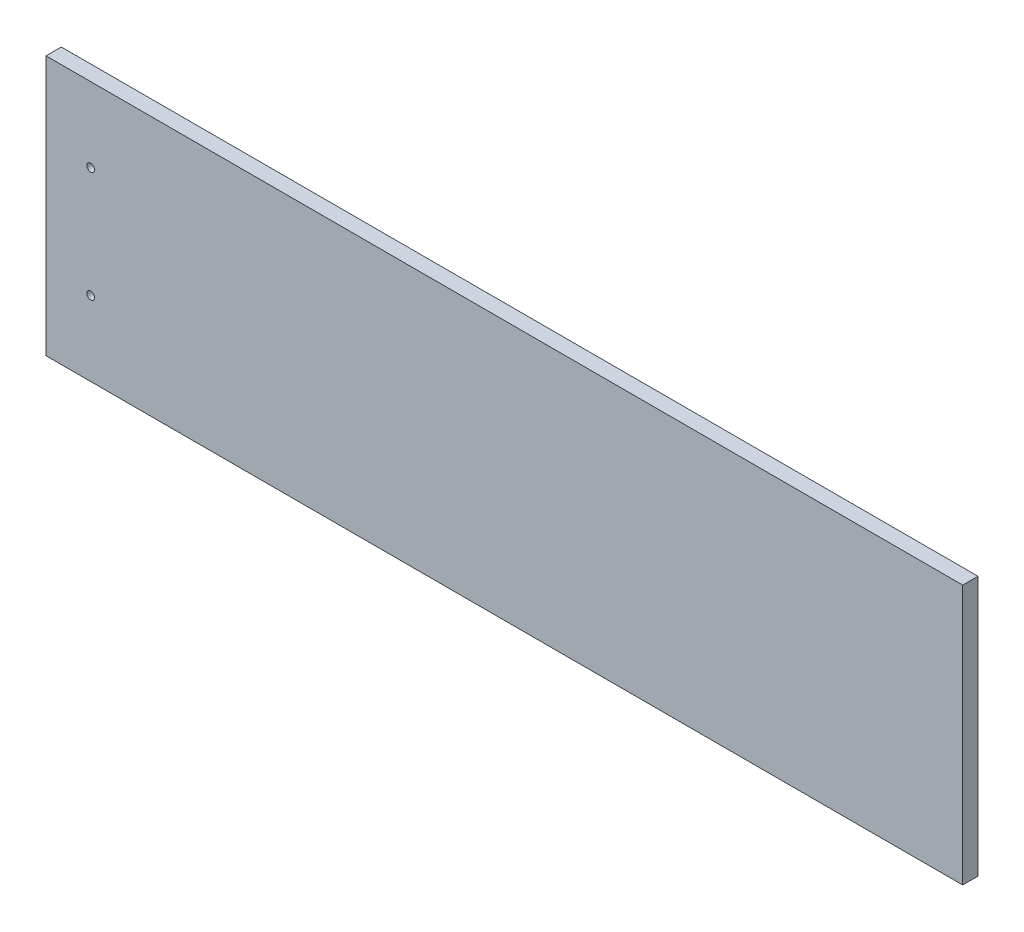
SolidWorks part; units mm, degrees
ref_plane "Front Plane" through (0, 0, 0) normal (0, 0, 1) x (1, 0, 0)
ref_plane "Top Plane" through (0, 0, 0) normal (0, 1, 0) x (1, 0, 0)
ref_plane "Right Plane" through (0, 0, 0) normal (1, 0, 0) x (0, 0, -1)
sketch "Sketch1" plane through (0, 0, 0) normal (0, 0, 1) x (1, 0, 0)
  line L1 (-300, 85) -> (300, 85)
  line L2 (-300, 85) -> (-300, -85)
  line L3 (-300, -85) -> (300, -85)
  line L4 (300, 85) -> (300, -85)
  line L5 (-300, 85) -> (300, -85) construction
  line L6 (-300, -85) -> (300, 85) construction
  point P0 (0, 0)
  dimension "D1" = 600
  dimension "D2" = 170
extrude "Boss-Extrude1" add sketch "Sketch1" along normal blind 10
hole_wizard "M6 Tapped Hole1" positions "Sketch2" profile "Sketch3" tap size "M6" standard "GB"
sketch "Sketch2" plane through (0, 0, 0) normal (0, 0, -1) x (-1, 0, 0)
  point P0 (270.75, 36.25)
  point P3 (270.75, -36.25)
sketch "Sketch3" plane through (-270.75, 36.25, 0) normal (1, 0, 0) x (0, 1, 0)
  line L0 (0, 0) -> (0, 16.5022)
  line L1 (0, 16.5022) -> (2.5, 15)
  line L2 (2.5, 15) -> (2.5, 0)
  line L5 (2.5, 0) -> (0, 0)
  line L10 (0, 16.5022) -> (-2.5, 15) construction
  line L11 (0, -6.35) -> (0, 107.95) construction
  dimension "螺纹孔钻头直径" = 5
  dimension "螺纹孔钻头深度" = 15
  dimension "导头角度" = 118
cosmetic thread "Cosmetic Thread1"
cosmetic thread "Cosmetic Thread2"
